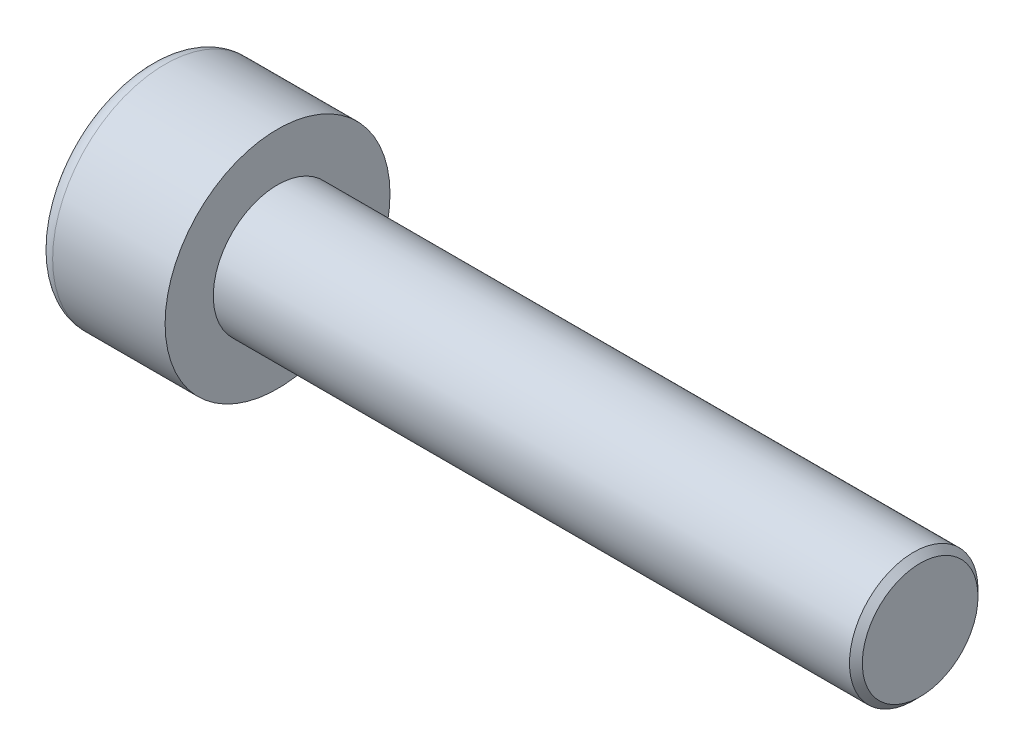
SolidWorks part; units mm, degrees
material "316L"
ref_plane "Front" through (0, 0, 0) normal (0, 0, 1) x (1, 0, 0)
ref_plane "Top" through (0, 0, 0) normal (0, 1, 0) x (1, 0, 0)
ref_plane "Right" through (0, 0, 0) normal (1, 0, 0) x (0, 0, -1)
sketch "Sketch1" plane through (0, 0, 0) normal (1, 0, 0) x (0, 0, -1)
  circle A0 centre (0, 0) radius 3.5
  dimension "dk" = 7
extrude "BaseHead" add sketch "Sketch1" along normal blind 4
sketch "Sketch2" plane through (4, 0, 0) normal (1, 0, 0) x (0, 0, -1)
  circle A0 centre (0, 0) radius 2
extrude "BaseBody" add sketch "Sketch2" along normal blind 20
cosmetic thread "ThreadCosmetic1" [suppressed] parameters "b"=16, "D2"=3.242
sketch "Sketch3" plane through (0, 0, 0) normal (1, 0, 0) x (0, 0, -1)
  line L1 (1.7321, 0) -> (0.866, 1.5)
  line L2 (0.866, 1.5) -> (-0.866, 1.5)
  line L3 (-0.866, 1.5) -> (-1.7321, 0)
  line L4 (-1.7321, 0) -> (-0.866, -1.5)
  line L5 (-0.866, -1.5) -> (0.866, -1.5)
  line L6 (0.866, -1.5) -> (1.7321, 0)
  circle A0 centre (0, 0) radius 1.5 construction
  dimension "s" = 3
  dimension "e" = 3.4641
extrude "HexagonSocket" cut sketch "Sketch3" along normal blind 2
sketch "Sketch4" plane through (-4.1961, 0.75, 0) normal (0, 0, 1) x (-1, 0, 0)
  line L0 (-6.1961, 2.25) -> (-7.0622, 0.75)
  line L2 (-7.0622, 0.75) -> (-6.1961, 0.75)
  line L3 (-6.1961, 0.75) -> (-6.1961, 2.25)
  line L4 (-5.0351, 0.75) -> (0.839, 0.75) construction
  line L5 (-28.1961, 0.75) -> (-8.1961, 0.75) construction
  line L6 (-8.1961, 0.75) -> (-4.1961, 0.75) construction
  dimension "m" = 60
revolve "Cut-Revolve1" cut sketch "Sketch4" angle 360 about L4
fillet "HeadFillet" [suppressed] radius 0.2
fillet "TopFillet" radius 0.5 1 edges at (0, 0, -3.5)
chamfer "Chamfer1" distance 0.2 angle 45 1 edges at (24, 0, -2)
sketch "Sketch5" plane through (0, 0, 0) normal (0, 0, 1) x (1, 0, 0)
  line L0 (23.8, 1.6718) -> (23.9895, 2)
  line L1 (23.9895, 2) -> (23.9895, 2.379)
  line L2 (23.9895, 2.379) -> (23.6105, 2.379)
  line L3 (23.6105, 2.379) -> (23.6105, 2)
  line L4 (23.6105, 2) -> (23.8, 1.6718)
  line L5 (0, 0) -> (7.8886, 0) construction
  line L6 (23.8, -2) -> (23.8, 2) construction
revolve "Cut-Revolve10" [suppressed] cut sketch "Sketch5" angle 360 about L5
pattern_linear "LPattern10" [suppressed] count 35 spacing 0.4548 along (1, 0, 0)
equation "\"r1@TopFillet\" = \"d@Sketch2\" / 8"
equation "\"D1@Chamfer1\" = \"r@HeadFillet\""
equation "\"D1@Sketch5\" = \"d@Sketch2\""
equation "\"D2@Sketch5\" =  ( \"d@Sketch2\" - \"D2@ThreadCosmetic1\" )  / 2"
equation "\"D3@LPattern10\" = \"D2@Sketch5\" * 1.2"
equation "\"D1@LPattern10\" = \"b@ThreadCosmetic1\" / \"D3@LPattern10\""
